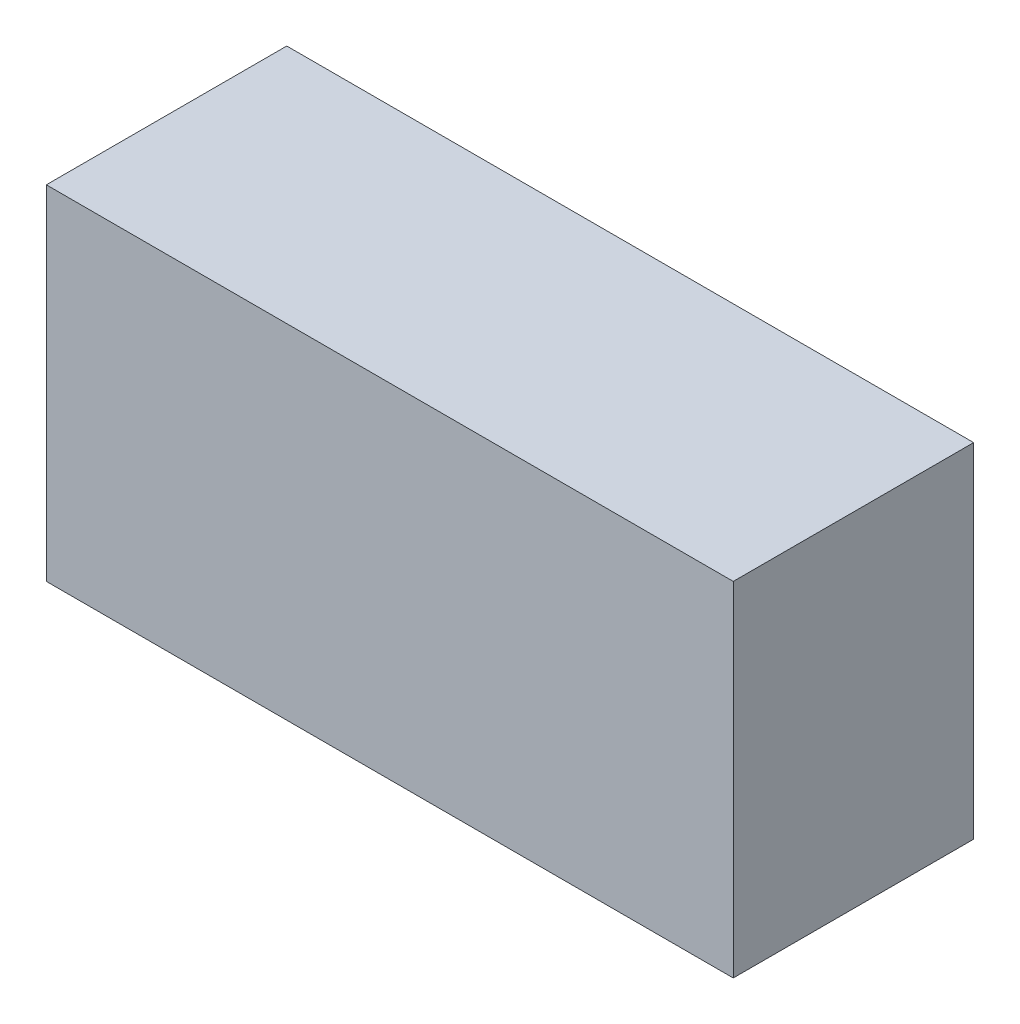
SolidWorks part; units mm, degrees
ref_plane "前视基准面" through (0, 0, 0) normal (0, 0, 1) x (1, 0, 0)
ref_plane "上视基准面" through (0, 0, 0) normal (0, 1, 0) x (1, 0, 0)
ref_plane "右视基准面" through (0, 0, 0) normal (1, 0, 0) x (0, 0, -1)
other "Configuration Table"
sketch "草图1" plane through (0, 0, 0) normal (0, 0, 1) x (1, 0, 0)
  line L0 (-10, -5) -> (10, -5)
  line L1 (10, -5) -> (10, 5)
  line L2 (10, 5) -> (-10, 5)
  line L3 (-10, 5) -> (-10, -5)
  point P0 (0, 0)
  dimension "D1" = 10
  dimension "D2" = 20
  dimension "D3" = 5
  dimension "D4" = 10
extrude "凸台-拉伸1" add sketch "草图1" against normal mid plane 7
